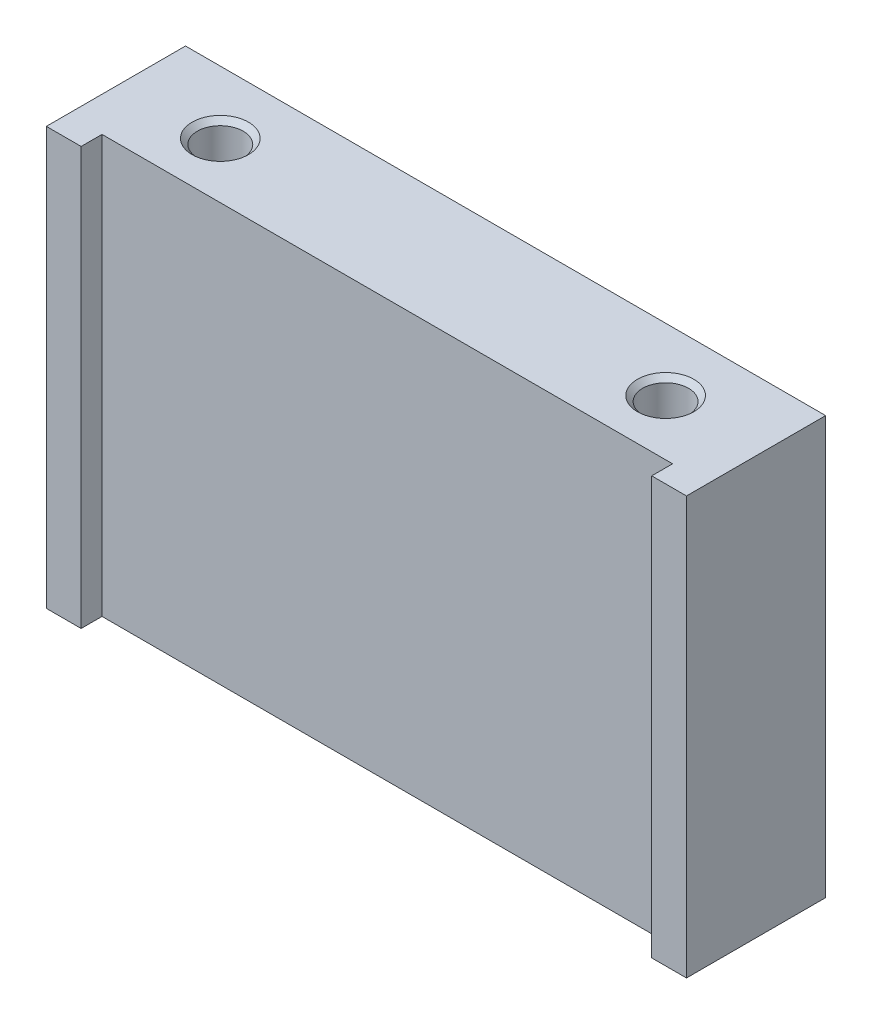
SolidWorks part; units mm, degrees
ref_plane "前视基准面" through (0, 0, 0) normal (0, 0, 1) x (1, 0, 0)
ref_plane "上视基准面" through (0, 0, 0) normal (0, 1, 0) x (1, 0, 0)
ref_plane "右视基准面" through (0, 0, 0) normal (1, 0, 0) x (0, 0, -1)
sketch "草图1" plane through (0, 0, 0) normal (0, 0, 1) x (1, 0, 0)
  line L1 (-23, -15) -> (23, -15)
  line L2 (-23, -15) -> (-23, 15)
  line L3 (-23, 15) -> (23, 15)
  line L4 (23, -15) -> (23, 15)
  line L5 (-23, -15) -> (23, 15) construction
  line L6 (-23, 15) -> (23, -15) construction
  point P0 (0, 0)
  dimension "D1" = 46
  dimension "D2" = 30
extrude "凸台-拉伸1" add sketch "草图1" along normal blind 10
sketch "草图2" plane through (0, 0, 10) normal (0, 0, 1) x (1, 0, 0)
  line L0 (-23, -15) -> (23, -15) construction
  line L1 (-20.5, 15) -> (20.5, 15)
  line L2 (-20.5, 15) -> (-20.5, -15)
  line L3 (-20.5, -15) -> (20.5, -15)
  line L4 (20.5, 15) -> (20.5, -15)
  line L5 (-20.5, 15) -> (20.5, -15) construction
  line L6 (-20.5, -15) -> (20.5, 15) construction
  line L7 (23, 15) -> (-23, 15) construction
  point P0 (0, 0)
  dimension "D1" = 41
extrude "切除-拉伸1" cut sketch "草图2" against normal blind 1.5
hole_wizard "M4 螺纹孔1" positions "3D草图1" profile "草图3" tap size "M4" standard "GB"
sketch3d "3D草图1"
  line L0 (20.5, 15, 8.5) -> (-20.5, 15, 8.5) construction
  line L1 (23, 15, 10) -> (23, 15, 0) construction
  point P0 (16, 15, 4.5)
  dimension "D1" = 4
  dimension "D2" = 7
sketch "草图3" plane through (16, 15, 4.5) normal (1, 0, 0) x (0, 0, 1)
  line L0 (0, 0) -> (0, 9.0914)
  line L1 (0, 9.0914) -> (1.65, 8.1)
  line L2 (1.65, 8.1) -> (1.65, 0.375)
  line L3 (1.65, 0.375) -> (2.025, 0)
  line L5 (2.025, 0) -> (0, 0)
  line L6 (-1.65, 0.375) -> (-2.025, 0) construction
  line L10 (0, 9.0914) -> (-1.65, 8.1) construction
  line L11 (0, -6.35) -> (0, 107.95) construction
  dimension "螺纹孔钻头直径" = 3.3
  dimension "螺纹孔钻头深度" = 8.1
  dimension "近端锥形沉头孔直径" = 4.05
  dimension "近端锥形沉头孔角度" = 90
  dimension "导头角度" = 118
cosmetic thread "孔螺蚊线1" parameters "D1"=6, "D2"=4
mirror "镜向1" about plane through (0, 0, 0) normal (1, 0, 0) of "M4 螺纹孔1"
